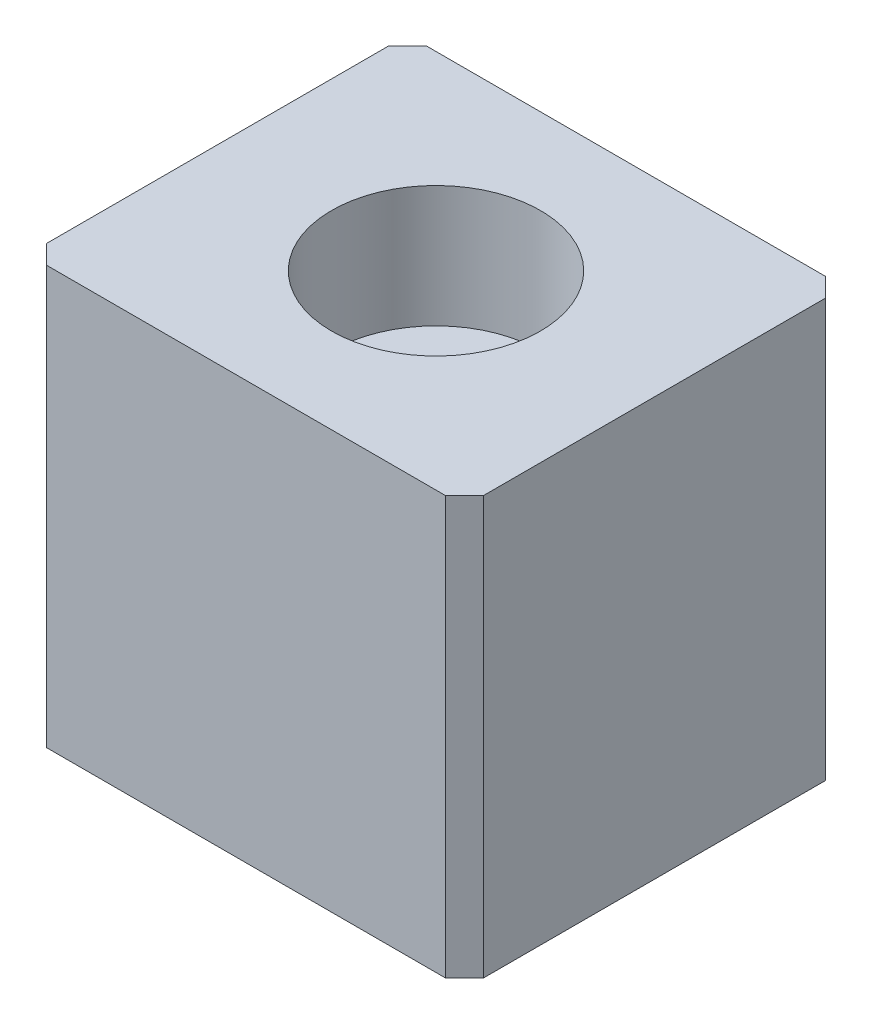
from build123d import *

# Parameters (mm, degrees)
SKETCH_1_W                   = 23
SKETCH_1_H                   = 20
EXTRUDE_1_DEPTH              = 11
HOLE_WIZARD_M6_1_D           = 6.6
HOLE_WIZARD_M6_1_CBORE_D     = 11
HOLE_WIZARD_M6_1_CBORE_DEPTH = 6.4
CHAMFER_1_SIZE               = 1


with BuildPart() as part:
    # 草图1 → 凸台-拉伸1 (new, symmetric)
    with BuildSketch(Plane(origin=(0, 0, 0), x_dir=(1, 0, 0), z_dir=(0, 1, 0))):
        Rectangle(SKETCH_1_W, SKETCH_1_H)
    extrude(amount=EXTRUDE_1_DEPTH, both=True)

    # M6 六角凹头螺钉的柱形沉头孔1 (through all)
    with Locations(Plane(origin=(0, 11, 0), x_dir=(1, 0, 0), z_dir=(0, 1, 0))):
        with Locations((0, 0)):
            CounterBoreHole(HOLE_WIZARD_M6_1_D / 2, HOLE_WIZARD_M6_1_CBORE_D / 2, HOLE_WIZARD_M6_1_CBORE_DEPTH)

    # 倒角1
    chamfer_1_edges = [part.edges().sort_by_distance(p)[0] for p in [
        (-11.5, 0, -10),
        (11.5, 0, -10),
        (11.5, 0, 10),
        (-11.5, 0, 10),
    ]]
    chamfer(chamfer_1_edges, length=CHAMFER_1_SIZE)


solid = part.part
